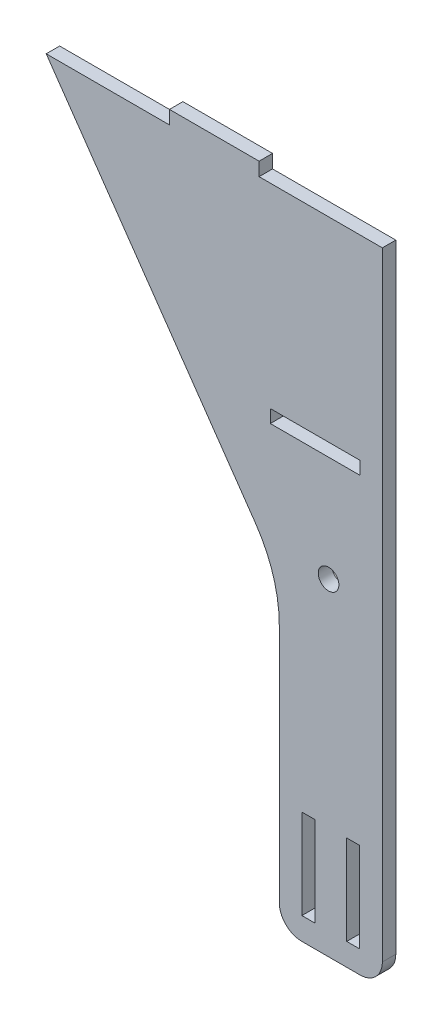
SolidWorks part; units mm, degrees
ref_plane "Front Plane" through (0, 0, 0) normal (0, 0, 1) x (1, 0, 0)
ref_plane "Top Plane" through (0, 0, 0) normal (0, 1, 0) x (1, 0, 0)
ref_plane "Right Plane" through (0, 0, 0) normal (1, 0, 0) x (0, 0, -1)
sketch "Sketch1" plane through (0, 0, 0) normal (0, 0, 1) x (1, 0, 0)
  line L0 (-6.5, 25) -> (-6.5, 5) construction
  line L1 (0, 0) -> (-23, 0)
  line L2 (0, 0) -> (0, 143)
  line L3 (0, 143) -> (-27.5, 143)
  line L4 (-23, 0) -> (-23, 68)
  line L5 (-16.5, 25) -> (-16.5, 5) construction
  line L11 (-17.95, 25) -> (-15.05, 25)
  line L12 (-17.95, 25) -> (-17.95, 5)
  line L13 (-17.95, 5) -> (-15.05, 5)
  line L14 (-15.05, 25) -> (-15.05, 5)
  line L17 (-7.95, 5) -> (-5.05, 5)
  line L18 (-7.95, 5) -> (-7.95, 25)
  line L19 (-7.95, 25) -> (-5.05, 25)
  line L20 (-5.05, 5) -> (-5.05, 25)
  line L25 (-23, 68) -> (-75, 143)
  line L26 (-47.5, 143) -> (-47.5, 146)
  line L27 (-47.5, 146) -> (-27.5, 146)
  line L28 (-27.5, 143) -> (-27.5, 146)
  line L30 (-75, 143) -> (-47.5, 143)
  dimension "D2" = 10
  dimension "D3" = 6.5
  dimension "D4" = 27.5
  dimension "D5" = 23
  dimension "D6" = 47.5
  dimension "D7" = 5
  dimension "D8" = 146
  dimension "D9" = 68
  dimension "D10" = 143
  dimension "D11" = 2.9
extrude "Boss-Extrude1" add sketch "Sketch1" along normal blind 3
fillet "Fillet1" radius 5 2 edges at (0, 0, 1.5) (-23, 0, 1.5)
fillet "Fillet2" radius 30 1 edges at (-23, 68, 1.5)
sketch "Sketch4" plane through (0, 0, 3) normal (0, 0, 1) x (1, 0, 0)
  line L0 (0, 5) -> (0, 143) construction
  line L1 (-18, 0) -> (-5, 0) construction
  circle A0 centre (-12, 73) radius 2.3
  dimension "D1" = 4.6
  dimension "D2" = 12
  dimension "D3" = 73
extrude "Cut-Extrude1" cut sketch "Sketch4" against normal blind 10
sketch "Sketch5" plane through (0, 0, 0) normal (0, 0, -1) x (-1, 0, 0)
  line L0 (5, 98) -> (25, 98) construction
  line L1 (5, 99.45) -> (25, 99.45)
  line L2 (5, 99.45) -> (5, 96.55)
  line L3 (5, 96.55) -> (25, 96.55)
  line L4 (25, 99.45) -> (25, 96.55)
  line L5 (0, 5) -> (0, 143) construction
  circle A0 centre (12, 73) radius 2.3 construction
  dimension "D1" = 20
  dimension "D2" = 2.9
  dimension "D3" = 25
  dimension "D4" = 5
extrude "Cut-Extrude2" cut sketch "Sketch5" against normal through all
